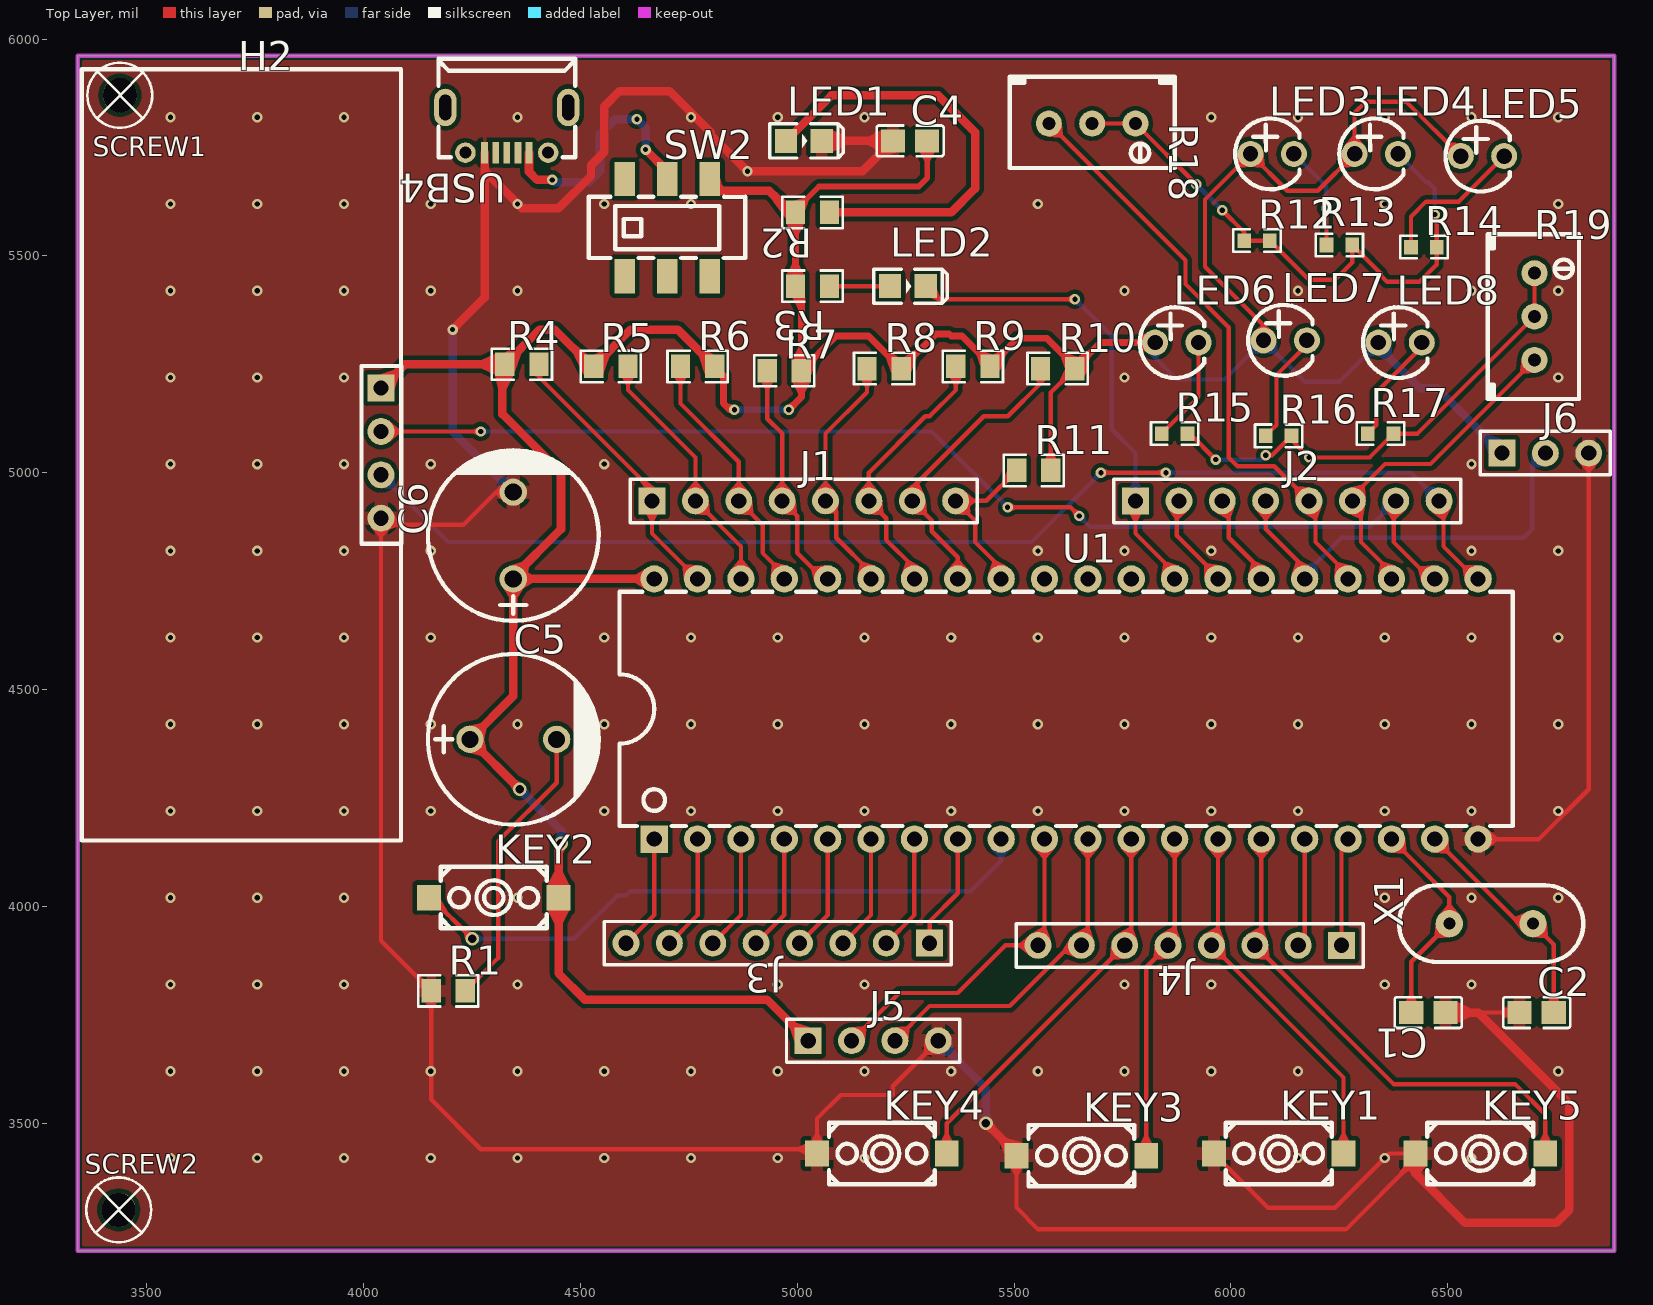
[diagram p0: Top Layer view]
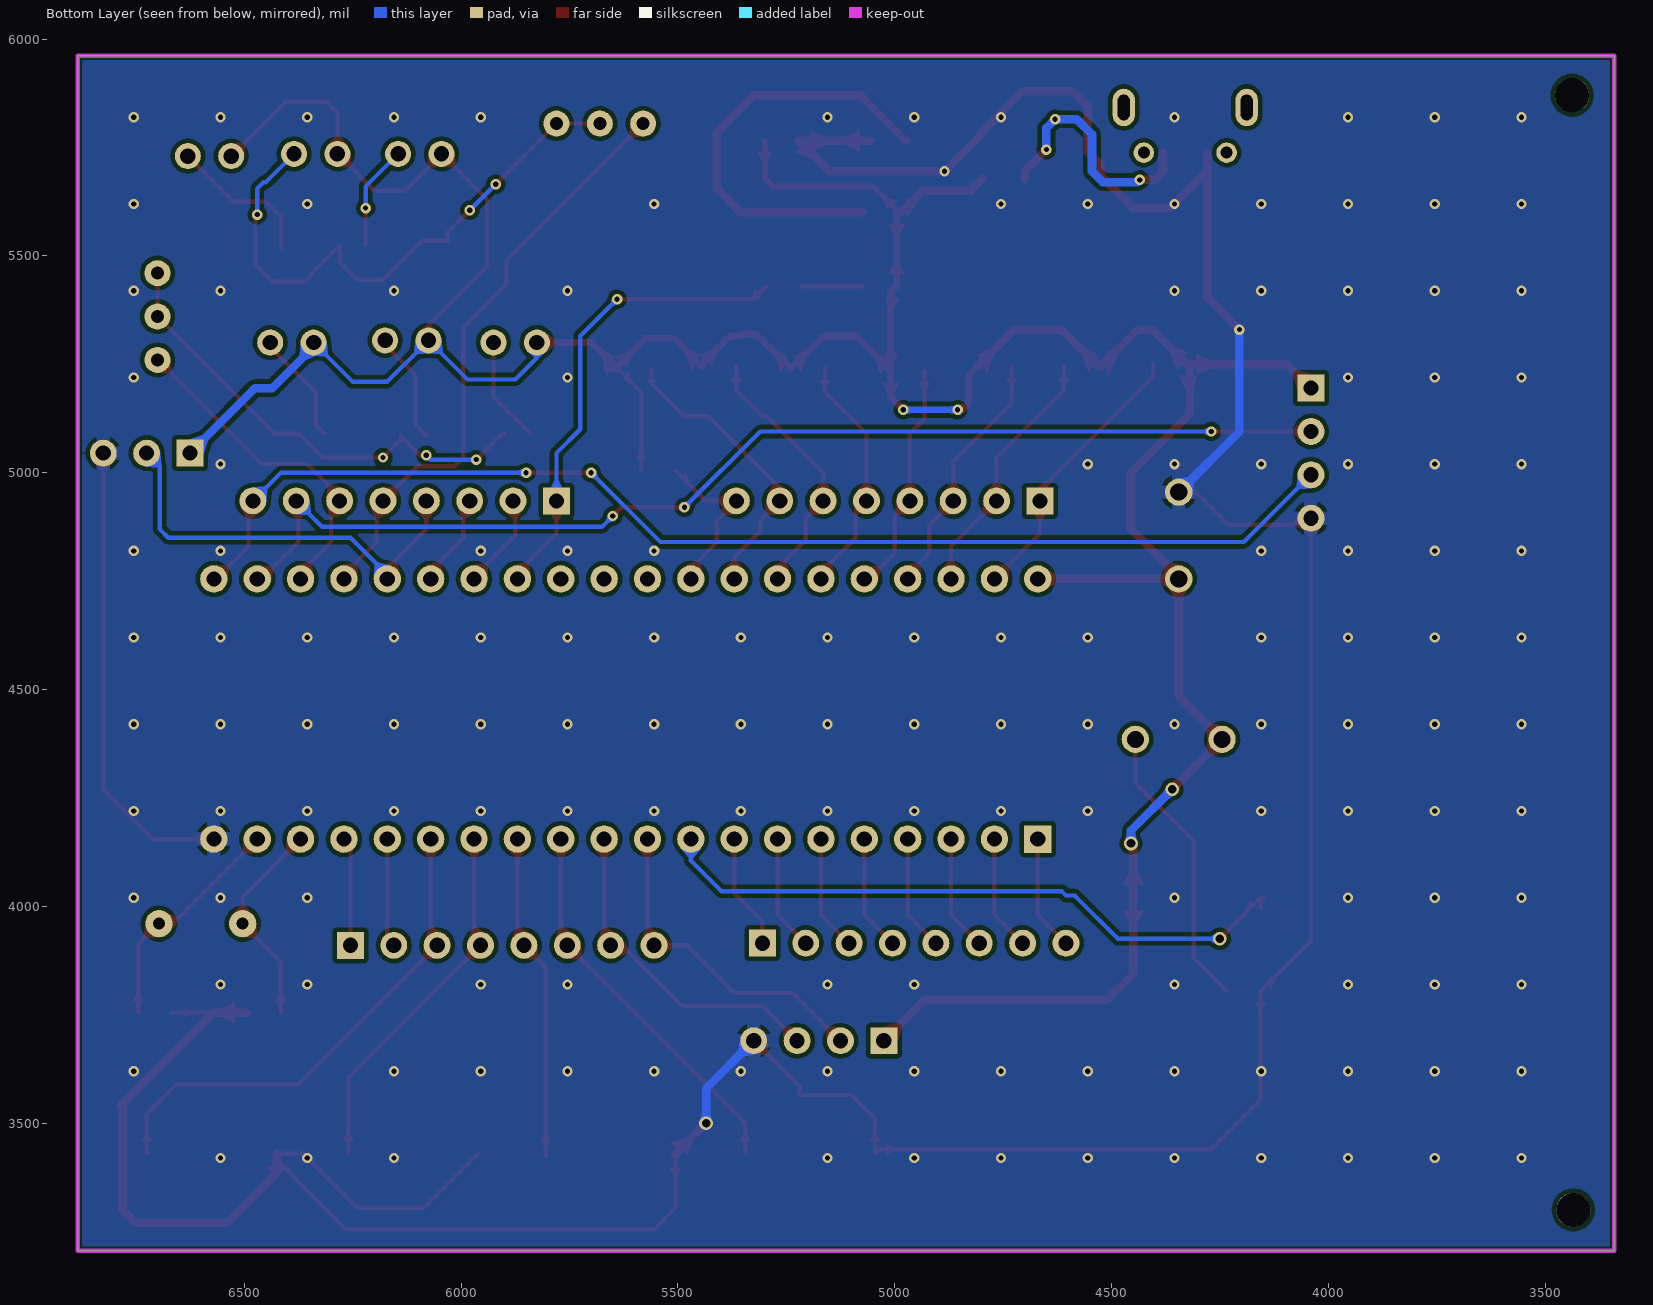
[diagram p1: Bottom Layer view, seen from below]
# Altium PCB MISC49914.pcbdoc
Units mil, origin at the board's own origin, x right, y up, seen from the top; angles counter-clockwise.
Board outline 3543.3 x 2755.9 mil, 2 copper layers (Top Layer, Bottom Layer), stack 62.206 mil thick; 50 components, 48 nets, 178 pads, 169 vias.

## Layer stack, top to bottom
Top Solder Mask Layer: solder mask 0.394, Dk 3.3
Top Layer: signal copper 1.379
Dielectric1: surface 59.449, FR4, Dk 4.5
Bottom Layer: signal copper 1.378
Bottom Solder Mask Layer: solder mask 0.394, Dk 3.3

## Board outline
3340.59,3205.55 3340.59,5961.45 6883.89,5961.45 6883.89,3205.55

## Design rules (kind name [scope] priority, off if disabled: settings)
BoardOutlineClearance Power_1 [All] p2 off: genericclearance=11.81 ignorepadtopadclearanceinfootprint=FALSE except(0: Text-CutoutEdge Arc-SplitContinuation Track-SplitContinuation SMDPad-SplitContinuation THPad-SplitContinuation Via-SplitContinuation Fill-SplitContinuation Region-SplitContinuation Poly-SplitContinuation Text-SplitContinuation Hole-SplitContinuation; 5.98: Arc-OutlineEdge Track-OutlineEdge SMDPad-OutlineEdge THPad-OutlineEdge Via-OutlineEdge Fill-OutlineEdge Region-OutlineEdge Text-OutlineEdge Hole-OutlineEdge; 10: Poly-OutlineEdge Poly-CutoutEdge; 11.81: Arc-CutoutEdge Track-CutoutEdge SMDPad-CutoutEdge THPad-CutoutEdge Via-CutoutEdge Fill-CutoutEdge Region-CutoutEdge Hole-CutoutEdge)
BoardOutlineClearance Plane_Default_1 [All] p4 off: genericclearance=5.98 ignorepadtopadclearanceinfootprint=FALSE except(0: Text-CutoutEdge Arc-SplitContinuation Track-SplitContinuation SMDPad-SplitContinuation THPad-SplitContinuation Via-SplitContinuation Fill-SplitContinuation Region-SplitContinuation Poly-SplitContinuation Text-SplitContinuation Hole-SplitContinuation; 5.98: Arc-OutlineEdge Track-OutlineEdge SMDPad-OutlineEdge THPad-OutlineEdge Via-OutlineEdge Fill-OutlineEdge Region-OutlineEdge Poly-OutlineEdge Text-OutlineEdge Hole-OutlineEdge Arc-CutoutEdge Track-CutoutEdge SMDPad-CutoutEdge THPad-CutoutEdge Via-CutoutEdge Fill-CutoutEdge Region-CutoutEdge Poly-CutoutEdge Hole-CutoutEdge)
BoardOutlineClearance Plane_Power_1 [All] p6 off: genericclearance=5.98 ignorepadtopadclearanceinfootprint=FALSE except(0: Text-CutoutEdge Arc-SplitContinuation Track-SplitContinuation SMDPad-SplitContinuation THPad-SplitContinuation Via-SplitContinuation Fill-SplitContinuation Region-SplitContinuation Poly-SplitContinuation Text-SplitContinuation Hole-SplitContinuation; 5.98: Arc-OutlineEdge Track-OutlineEdge SMDPad-OutlineEdge THPad-OutlineEdge Via-OutlineEdge Fill-OutlineEdge Region-OutlineEdge Poly-OutlineEdge Text-OutlineEdge Hole-OutlineEdge Arc-CutoutEdge Track-CutoutEdge SMDPad-CutoutEdge THPad-CutoutEdge Via-CutoutEdge Fill-CutoutEdge Region-CutoutEdge Poly-CutoutEdge Hole-CutoutEdge)
BoardOutlineClearance Copper_gge8343_1 [All] p8 off: genericclearance=5.98 ignorepadtopadclearanceinfootprint=FALSE except(0: Text-CutoutEdge Arc-SplitContinuation Track-SplitContinuation SMDPad-SplitContinuation THPad-SplitContinuation Via-SplitContinuation Fill-SplitContinuation Region-SplitContinuation Poly-SplitContinuation Text-SplitContinuation Hole-SplitContinuation; 5.98: Arc-OutlineEdge Track-OutlineEdge SMDPad-OutlineEdge THPad-OutlineEdge Via-OutlineEdge Fill-OutlineEdge Region-OutlineEdge Text-OutlineEdge Hole-OutlineEdge Arc-CutoutEdge Track-CutoutEdge SMDPad-CutoutEdge THPad-CutoutEdge Via-CutoutEdge Fill-CutoutEdge Region-CutoutEdge Hole-CutoutEdge; 10: Poly-OutlineEdge Poly-CutoutEdge)
BoardOutlineClearance Copper_gge8337_1 [All] p10 off: genericclearance=5.98 ignorepadtopadclearanceinfootprint=FALSE except(0: Text-CutoutEdge Arc-SplitContinuation Track-SplitContinuation SMDPad-SplitContinuation THPad-SplitContinuation Via-SplitContinuation Fill-SplitContinuation Region-SplitContinuation Poly-SplitContinuation Text-SplitContinuation Hole-SplitContinuation; 5.98: Arc-OutlineEdge Track-OutlineEdge SMDPad-OutlineEdge THPad-OutlineEdge Via-OutlineEdge Fill-OutlineEdge Region-OutlineEdge Text-OutlineEdge Hole-OutlineEdge Arc-CutoutEdge Track-CutoutEdge SMDPad-CutoutEdge THPad-CutoutEdge Via-CutoutEdge Fill-CutoutEdge Region-CutoutEdge Hole-CutoutEdge; 10: Poly-OutlineEdge Poly-CutoutEdge)
BoardOutlineClearance Default_1 [All] p12: genericclearance=5.98 ignorepadtopadclearanceinfootprint=FALSE except(0: Text-CutoutEdge Arc-SplitContinuation Track-SplitContinuation SMDPad-SplitContinuation THPad-SplitContinuation Via-SplitContinuation Fill-SplitContinuation Region-SplitContinuation Poly-SplitContinuation Text-SplitContinuation Hole-SplitContinuation; 5.98: Arc-OutlineEdge Track-OutlineEdge SMDPad-OutlineEdge THPad-OutlineEdge Via-OutlineEdge Fill-OutlineEdge Region-OutlineEdge Text-OutlineEdge Hole-OutlineEdge Arc-CutoutEdge Track-CutoutEdge SMDPad-CutoutEdge THPad-CutoutEdge Via-CutoutEdge Fill-CutoutEdge Region-CutoutEdge Hole-CutoutEdge; 10: Poly-OutlineEdge Poly-CutoutEdge)
Clearance Power [All] p1 off: gap=11.81 ignorepadtopadclearanceinfootprint=FALSE except(0: Text-Text; 10: Poly-Track Poly-SMDPad Poly-THPad Poly-Via Poly-Fill Poly-Region Poly-Poly Poly-Arc Poly-Text Poly-Hole)
Clearance Plane_Default [All] p3 off: gap=5.98 ignorepadtopadclearanceinfootprint=FALSE except(0: Text-Text)
Clearance Plane_Power [All] p5 off: gap=5.98 ignorepadtopadclearanceinfootprint=FALSE except(0: Text-Text; 11.81: Poly-Track Poly-SMDPad Poly-THPad Poly-Via Poly-Fill Poly-Region Poly-Poly Poly-Arc Poly-Text Poly-Hole)
Clearance Copper_gge8343 [All] p7 off: gap=5.98 ignorepadtopadclearanceinfootprint=FALSE except(0: Text-Text; 10: Poly-Track Poly-SMDPad Poly-THPad Poly-Via Poly-Fill Poly-Region Poly-Poly Poly-Arc Poly-Text Poly-Hole)
Clearance Copper_gge8337 [All] p9 off: gap=5.98 ignorepadtopadclearanceinfootprint=FALSE except(0: Text-Text; 10: Poly-Track Poly-SMDPad Poly-THPad Poly-Via Poly-Fill Poly-Region Poly-Poly Poly-Arc Poly-Text Poly-Hole)
Clearance Default [All] p11: gap=5.98 ignorepadtopadclearanceinfootprint=FALSE except(0: Text-Text; 10: Poly-Track Poly-SMDPad Poly-THPad Poly-Via Poly-Fill Poly-Region Poly-Poly Poly-Arc Poly-Text Poly-Hole)
DiffPairsRouting differentialPair [All] p1: maxlimit=6 minlimit=6 mostfreqgap=6 toplayer_minwidth=5 toplayer_prefwidth=10 toplayer_maxwidth=100 toplayer_mingap=6 toplayer_prefgap=6 toplayer_maxgap=6 bottomlayer_minwidth=5 bottomlayer_prefwidth=10 bottomlayer_maxwidth=100 bottomlayer_mingap=6 bottomlayer_prefgap=6 bottomlayer_maxgap=6 maxuncoupledlength=10
HoleToHoleClearance otherClearance [All] p1: gap=11.8 allowstackedmicrovias=TRUE
Length netLength [All] p1: minlimit=0 maxlimit=0
PasteMaskExpansion pasteMaskExpansion [All] p1: expansion=0
PlaneConnect Power_4 [All] p1 off: planeconnectstyle=Relief reliefexpansion=20 reliefentries=4 reliefconductorwidth=0 reliefairgap=10
PlaneConnect Default_4 [All] p2: planeconnectstyle=Relief reliefexpansion=20 reliefentries=4 reliefconductorwidth=0 reliefairgap=10
PolygonConnect gge8337 [All] p1 off: connectstyle=Relief reliefconductorwidth=0 reliefentries=4 polygonreliefangle="90 Angle" airgapwidth=10 via.connectstyle=Relief via.reliefconductorwidth=10 via.reliefentries=4 via.polygonreliefangle="90 Angle" via.airgapwidth=10
PolygonConnect gge8343 [All] p2: connectstyle=Relief reliefconductorwidth=0 reliefentries=4 polygonreliefangle="90 Angle" airgapwidth=10 via.connectstyle=Relief via.reliefconductorwidth=10 via.reliefentries=4 via.polygonreliefangle="90 Angle" via.airgapwidth=10
RoutingVias Power_3 [All] p1 off: holewidth=11.81 width=23.62 viastyle="Through Hole" minholewidth=11.81 minwidth=23.62 maxholewidth=2362 maxwidth=3938
RoutingVias Default_3 [All] p2: holewidth=12.01 width=23.62 viastyle="Through Hole" minholewidth=12.01 minwidth=23.62 maxholewidth=2362 maxwidth=3938
SolderMaskExpansion solderMaskExpansion [IsVia] p1: expansion=-1000 istentingtop=TRUE
SolderMaskExpansion solderMaskExpansion [All] p2: expansion=2 istentingtop=FALSE
Width Power_2 [All] p1 off: maxlimit=1000 minlimit=19.7 preferedwidth=19.7
Width Default_2 [All] p2: maxlimit=1000 minlimit=10 preferedwidth=10

## Components (designator, comment, footprint, x,y, rotation, side; value= is the part's Value field where it differs from the comment)
C1 "33p" C0805 6455,3755 r180 top
C2 "33p" C0805 6705,3755 r0 top
C4 "10NF" C0805 5260,5765 r0 top
C5 "10uF" CAP-TH_BD10.0-P5.00-D1.0-FD 4345,4385 r0 top
C6 "10uF" CAP-TH_BD10.0-P5.00-D1.0-FD 4345,4855 r90 top
H2 "HC-SR04" HC-SR04 4040,5045 r0 top
J1 "HDR-M-2.54_1x8" HDR-M-2.54_1X8 5065,4935 r0 top
J2 "HDR-M-2.54_1x8" HDR-M-2.54_1X8 6180,4935 r0 top
J3 "HDR-M-2.54_1x8" HDR-M-2.54_1X8 4905,3915 r180 top
J4 "HDR-M-2.54_1x8" HDR-M-2.54_1X8 5855,3910 r180 top
J5 "HDR-M-2.54_1x4" HDR-M-2.54_1X4 5175,3690 r0 top
J6 "HDR-M-2.54_1x3" HDR-M-2.54_1X3 6725,5045 r0 top
KEY1 "K2-3.6×6.1_SMD" KEY-SMD_2P-L6.2-W3.6-LS8.0 6110,3430 r0 top
KEY2 "K2-3.6×6.1_SMD" KEY-SMD_2P-L6.2-W3.6-LS8.0 4300,4020 r0 top
KEY3 "K2-3.6×6.1_SMD" KEY-SMD_2P-L6.2-W3.6-LS8.0 5655,3425 r0 top
KEY4 "K2-3.6×6.1_SMD" KEY-SMD_2P-L6.2-W3.6-LS8.0 5195,3430 r0 top
KEY5 "K2-3.6×6.1_SMD" KEY-SMD_2P-L6.2-W3.6-LS8.0 6575,3430 r0 top
LED1 "LED-0805_R" LED0805_RED 5015,5765 r0 top
LED2 "LED-0805_R" LED0805_RED 5255,5430 r0 top
LED3 "204-10SDRD/S530-A3-L" LED-TH_BD3.8-P2.54-FD 6095,5735 r0 top
LED4 "204-10SDRD/S530-A3-L" LED-TH_BD3.8-P2.54-FD 6335,5735 r0 top
LED5 "204-10SDRD/S530-A3-L" LED-TH_BD3.8-P2.54-FD 6580,5730 r0 top
LED6 "204-10SDRD/S530-A3-L" LED-TH_BD3.8-P2.54-FD 5875,5300 r0 top
LED7 "204-10SDRD/S530-A3-L" LED-TH_BD3.8-P2.54-FD 6125,5305 r0 top
LED8 "204-10SDRD/S530-A3-L" LED-TH_BD3.8-P2.54-FD 6390,5300 r0 top
R1 "10k" R0805 4195,3805 r0 top
R2 "1.5k" R0805 5035,5600 r180 top
R3 "1k" R0805 5035,5430 r180 top
R4 "4.7k" R0805 4365,5250 r180 top
R5 "4.7k" R0805 4570,5245 r180 top
R6 "4.7k" R0805 4770,5245 r0 top
R7 "4.7k" R0805 4970,5235 r0 top
R8 "4.7k" R0805 5200,5240 r0 top
R9 "4.7k" R0805 5405,5245 r0 top
R10 "4.7k" R0805 5600,5240 r0 top
R11 "4.7k" R0805 5545,5005 r0 top
R12 "1000" R0603 6060,5535 r0 top
R13 "1000" R0603 6250,5525 r0 top
R14 "1000" R0603 6445,5520 r0 top
R15 "1000" R0603 5870,5090 r0 top
R16 "1000" R0603 6110,5085 r0 top
R17 "1000" R0603 6345,5090 r0 top
R18 "10kΩ" RES-ADJ-TH_3296W 5680,5805 r270 top
R19 "10kΩ" RES-ADJ-TH_3296W 6700,5360 r0 top
SCREW1 "" M2螺丝 3437.7,5870.25 r0 top
SCREW2 "" M2螺丝 3435,3300 r0 top
SW2 "MST22D18G2 125" SW-SMD_MST22D18G2 4700,5565 r0 top
U1 "STC90C52RC-40I_C14023" DIP-40_L52.0-W13.7-P2.54-LS15.2-BL 5620,4455 r0 top
USB4 "USB-Micro_1" MICRO-USB-SMD_5P-P0.65-H-F_C10418 4330,5790 r180 top
X1 "11.0592MHz" OSC-TH_L10.0-W4.5-P5.00 6600,3960 r90 top

## Footprints (in the part's own frame and the unit in brackets; to place one, negate y for a bottom-side part, rotate by r counter-clockwise, add the part's x,y. Pads: shape width x height; smd on the part's side, far side on the other; paste and mask are expansions set on the pad)
C0805 [mm]
  rect 1.41x1.35 smd paste-100 mask+0.051: 1(-1,0) 2(1,0)
  silkscreen extent -1.96,-0.9 1.96,0.9
CAP-TH_BD10.0-P5.00-D1.0-FD [mm]
  round 1.6 hole 1 paste+0 mask+0.051: 1(-2.54,0) 2(2.54,0)
  silkscreen extent -5,-5 5.08,5
DIP-40_L52.0-W13.7-P2.54-LS15.2-BL [mil]
  rect 63x63 hole 35 paste+0 mask+2: 1(-950,-300)
  round 63 hole 35 paste+0 mask+2: 2(-850,-300) 3(-750,-300) 4(-650,-300) 5(-550,-300) 6(-450,-300) 7(-350,-300) 8(-250,-300) 9(-150,-300) 10(-50,-300) 11(50,-300) 12(150,-300) 13(250,-300) 14(350,-300) 15(450,-300) 16(550,-300) 17(650,-300) 18(750,-300) 19(850,-300) 20(950,-300) 21(950,300) 22(850,300) 23(750,300) 24(650,300) 25(550,300) 26(450,300) 27(350,300) 28(250,300) 29(150,300) 30(50,300) 31(-50,300) 32(-150,300) 33(-250,300) 34(-350,300) 35(-450,300) 36(-550,300) 37(-650,300) 38(-750,300) 39(-850,300) 40(-950,300)
  silkscreen extent -1030,-270 1030,270
HC-SR04 [mil]
  rect 62x62 hole 35 paste+0 mask+2: 1(0,150)
  round 62 hole 35 paste+0 mask+2: 2(0,50) 3(0,-50) 4(0,-150)
  silkscreen extent -690,-893 47,885
HDR-M-2.54_1X3 [mil]
  rect 62x62 hole 35 paste+0 mask+2: 1(-100,0)
  round 62 hole 35 paste+0 mask+2: 2(0,0) 3(100,0)
  silkscreen extent -150,-50 150,50
HDR-M-2.54_1X4 [mil]
  rect 62x62 hole 35 paste+0 mask+2: 1(-150,0)
  round 62 hole 35 paste+0 mask+2: 2(-50,0) 3(50,0) 4(150,0)
  silkscreen extent -200,-50 200,50
HDR-M-2.54_1X8 [mil]
  rect 62x62 hole 35 paste+0 mask+2: 1(-400,0)
  round 62 hole 35 paste+0 mask+2: 2(-300,0) 3(-200,0) 4(-100,0) 5(0,0) 6(100,0) 7(200,0) 8(300,0)
  silkscreen extent -450,-50 350,50
KEY-SMD_2P-L6.2-W3.6-LS8.0 [mm]
  rect 1.4x1.5 smd paste+0 mask+0.051: 1(-3.8,0) 2(3.8,0)
  silkscreen extent -3.1,-1.8 3.1,1.8
LED0805_RED [mil]
  rect 51.2x55.1 smd paste+0 mask+2: 1(-41.35,0) 2(41.35,0)
  silkscreen extent -79,-39 91,39
LED-TH_BD3.8-P2.54-FD [mil]
  round 60 hole 35.43 paste+0 mask+2: 1(-50,0) 2(50,0)
  silkscreen extent -85,-82 63,82
M2螺丝 [mm]
  round 2 hole 2: 1(0,0)
  silkscreen extent -1.9,-1.9 1.9,1.9
MICRO-USB-SMD_5P-P0.65-H-F_C10418 [mm]
  rect 0.4x1.25 smd paste-100 mask+0.051: 1(-1.3,1.325) 2(-0.65,1.325) 3(0,1.325) 4(0.65,1.325) 5(1.3,1.325)
  round 1.2 hole 0.7 paste+0 mask+0.051: SH0(-2.425,1.325) SH3(2.425,1.325)
  oval 1.3x2.2 hole 0.7 slot 1.5 at 90 deg paste+0 mask+0.051: SH1(-3.6,-1.325) SH2(3.6,-1.325)
  silkscreen extent -4,-4.17 4,1.59
OSC-TH_L10.0-W4.5-P5.00 [mm]
  round 1.6 hole 0.7 paste+0 mask+0.051: 1(0,2.45) 2(0,-2.45)
  silkscreen extent -2.25,-5.39 2.25,5.39
R0603 [mil]
  rect 31.75x34.02 smd paste-3937.01 mask+2: 1(-29.66,0) 2(29.66,0)
  silkscreen extent -55,-26 55,26
R0805 [mm]
  rect 1.133x1.377 smd paste-100 mask+0.051: 1(-1,0) 2(1,0)
  silkscreen extent -1.76,-0.92 1.76,0.92
RES-ADJ-TH_3296W [mil]
  round 60 hole 30 paste+0 mask+2: 1(0,99.99) 2(0,-0.01) 3(0,-100.01)
  silkscreen extent -108,-190 102,190
SW-SMD_MST22D18G2 [mm]
  rect 1.2x2 smd paste+0 mask+0.051: 1(-2.5,2.85) 2(0,2.85) 3(2.5,2.85) 4(-2.5,-2.85) 5(0,-2.85) 6(2.5,-2.85)
  silkscreen extent -4.6,-1.78 4.57,1.8

## Via types
v1: diameter 23.62, hole 12, Top Layer to Bottom Layer, 145 vias
v2: diameter 24, hole 12, Top Layer to Bottom Layer, 20 vias
v3: diameter 31.5, hole 19.7, Top Layer to Bottom Layer, 4 vias

## Nets (pads, with @x,y where several pads share a name; then routed paths per layer and width w, separated by ;. In a path a pad name is that pad's centre, name@x,y a point inside that pad or via, vN(x,y) a via of type N, cw(c..) or ccw(c..) an arc to the next point about the centre after c; other vN are vias at no path point)
$1N75: J3.8 U1.1 | length 266.9
  Top Layer w10: J3.8 4670,3980 U1.1
$1N76: J3.7 U1.2 | length 266.9
  Top Layer w10: J3.7 4770,3980 U1.2
$1N77: J3.6 U1.3 | length 266.9
  Top Layer w10: J3.6 4870,3980 U1.3
$1N78: J3.5 U1.4 | length 266.9
  Top Layer w10: J3.5 4970,3980 U1.4
$1N79: J3.4 U1.5 | length 266.9
  Top Layer w10: J3.4 5070,3980 U1.5
$1N80: J3.3 U1.6 | length 266.9
  Top Layer w10: J3.3 5170,3980 U1.6
$1N81: J3.2 U1.7 | length 266.9
  Top Layer w10: J3.2 5270,3980 U1.7
$1N82: J3.1 U1.8 | length 266.9
  Top Layer w10: J3.1 5305,3965 5370,4030 U1.8
$1N95: J4.2 U1.16 | length 251.2
  Top Layer w10: J4.2 6170,3925 U1.16
$1N96: J4.1 U1.17 | length 251.2
  Top Layer w10: J4.1 6255,4140 U1.17
$1N164: SW2.2 USB4.1 | length 579.3
  Top Layer w19.68: USB4.1 4381.2,5693.8 4400,5675 v2(4435,5675) ; v2(4650,5745) 4700,5695 SW2.2
  Bottom Layer w19.68: v2(4435,5675) 4440,5670 4520,5670 4545,5695 4545,5780 4580,5815 v2(4630,5815) 4650,5795 v2(4650,5745)
$1N297: LED1.1 R2.1 | length 1003.4
  Top Layer w19.68: LED1.1@4973.7,5765 5078.7,5870 5325,5870 5410,5785 5410,5655 5355,5600 R2.1
$1N368: LED2.1 R3.1 | length 139.3
  Top Layer w10: R3.1 LED2.1@5213.7,5430
$1N557: LED4.2 R12.1 R12.2 R13.2 R14.2 R18.1 R18.2 | length 1361.9
  Top Layer w10: R18.2 R18.1 v2(5920,5665) ; v2(5980,5605) 6030.3,5554.7 R12.1 R12.2 6179.7,5445 6240,5445 6279.7,5484.7 R13.2 6345,5459.7 6345,5455 6360,5440 6435,5440 6474.7,5479.7 R14.2 6474.7,5590.3 v2(6470,5595)
  Bottom Layer w10: v2(5920,5665) v2(5980,5605) ; LED4.2 6450,5670 6455,5670 6470,5655 v2(6470,5595)
$1N566: LED3.2 R13.1 | length 241.1
  Top Layer w10: v2(6220,5610) R13.1
  Bottom Layer w10: LED3.2 6220,5660 v2(6220,5610)
$1N604: LED5.2 R14.1 | length 342.9
  Top Layer w10: R14.1 6415.3,5590.3 6450,5625 6525,5625 LED5.2
$1N665: LED8.2 R17.1 | length 261.7
  Top Layer w10: R17.1 6335,5109.7 6335,5185 6440,5290 LED8.2
$1N666: LED7.2 R16.1 | length 259.2
  Top Layer w10: R16.1 6105,5109.7 6105,5225 6175,5295 LED7.2
$1N673: R15.2 R16.2 R17.2 R19.1 R19.2 | length 1108.9
  Top Layer w10: R15.2 5905,5090 v2(5965,5030) ; v2(6080,5040) 6094.7,5040 R16.2 6139.7,5075.3 v2(6180,5035) 6319.7,5035 R17.2 6430,5090 R19.2 R19.1
  Bottom Layer w10: v2(5965,5030) 6070,5030 v2(6080,5040)
$1N675: LED6.2 R15.1 | length 245.1
  Top Layer w10: R15.1 5925,5174.7 LED6.2
$1N776: C5.2 R1.2 | length 667.2
  Top Layer w10: R1.2 4310,3880.6 4310,4150 4445,4285 C5.2
+5V: C4.2 C5.1 C6.1 H2.1 J5.1 J6.1 KEY2.2 LED3.1 LED4.1 LED5.1 LED6.1 LED7.1 LED8.1 R2.2 R3.2 R4.2 R5.2 R6.2 R7.2 R8.2 R9.2 R10.2 R11.2 SW2.3 U1.40 | length 8572.5
  Top Layer w10: R11.2 5584.4,5185 R10.2 ; LED7.1 6075,5340 5940,5475 5940,5630 LED3.1 6130,5650 6200,5650 LED4.1 6285,5830 6310,5855 6405,5855 LED5.1
  Top Layer w13: R2.2 4995.6,5605.6 5050,5660 5280,5660 5300,5680 C4.2
  Top Layer w15.75: R6.2 4830,5224.4 4830,5160 4845,5145 v2(4855,5145) ; v2(4980,5145) 5009.4,5174.4 R7.2 ; R2.2 R3.2 5009.4,5416.3 R7.2 ; LED6.1 5699.4,5300 R10.2 5660,5240 5665,5245 5640,5245 5575,5310 5509.4,5310 R9.2 5444.4,5250.6 5380,5315 5355,5315 5350,5320 5319.4,5320 R8.2 5164.4,5315 5089.4,5315 R7.2
  Top Layer w19.68: H2.1 4095,5250 R4.2 ; v3(4360,4270) C5.1 4345,4485 C6.1 ; v3(4455,4145) 4449.6,4139.6 KEY2.2 4449.6,3845.4 4510,3785 4930,3785 J5.1 ; U1.40 C6.1 ; SW2.3 4825.6,5650 4935,5650 4985,5600 R2.2 ; R6.2 4724.4,5330 4615.6,5330 R5.2 4525,5245 4440,5330 4405.6,5330 R4.2 ; R4.2 4320,5244.4 4320,5135 4455,5000 4455,4870 4345,4760 C6.1
  Bottom Layer w10: LED6.1 5825,5265 5875,5215 5985,5215 LED7.1 6170,5210 6250,5210 LED8.1
  Bottom Layer w15.75: v2(4855,5145) v2(4980,5145)
  Bottom Layer w19.68: v3(4360,4270) 4455,4175 v3(4455,4145) ; LED8.1 6340,5290 6435,5195 6475,5195 J6.1
GND: C1.1 C2.1 C4.1 C6.2 H2.4 J5.4 J6.3 KEY1.1 KEY3.1 KEY4.1 KEY5.1 LED1.2 R1.1 U1.20 USB4.5 | length 9845
  Top Layer w10: C6.2 4305,4955 4230,4880 4055,4880 H2.4 4040,3920.6 R1.1 4155.6,3554.4 4270,3440 5035.4,3440 KEY4.1 5045.4,3510.4 5100,3565 5220,3565 5220,3585 J5.4 ; KEY3.1 5505.4,3305.4 5555,3255 6265,3255 6425.4,3415.4 KEY5.1 6365,3430 6354.67,3419.67 6240,3305 6085.4,3305 KEY1.1 ; C1.1 C2.1 ; U1.20@6575,4155 6710,4155 6825,4270 J6.3
  Top Layer w19.68: v2(4205,5330) 4278.8,5403.8 USB4.5 4278.8,5696.2 4365,5610 4450,5610 4525,5685 4525,5710 4555,5740 4555,5845 4590,5880 4705,5880 4800,5785 4800,5780 v2(4885,5695) 5150.6,5695 C4.1 LED1.2@5056.3,5765 ; v3(5435,3500) 5505.4,3429.6 KEY3.1 ; KEY5.1 6425.4,3384.6 6540,3270 6750,3270 6780,3300 6780,3535 6785,3540 6570,3755 C1.1
  Bottom Layer w19.68: v2(4205,5330) 4205,5095 C6.2 ; J5.4 5435,3580 v3(5435,3500)
  other v1: 3554.69,3419.65 3754.69,3419.65 3954.69,3419.65 4154.69,3419.65 4354.69,3419.65 4554.69,3419.65 4754.69,3419.65 4954.69,3419.65 5154.69,3419.65 6154.69,3419.65 6354.69,3419.65 6554.69,3419.65 3554.69,3619.65 3754.69,3619.65 3954.69,3619.65 4154.69,3619.65 4354.69,3619.65 4554.69,3619.65 4754.69,3619.65 4954.69,3619.65 5154.69,3619.65 5354.69,3619.65 5554.69,3619.65 5754.69,3619.65 5954.69,3619.65 6154.69,3619.65 6754.69,3619.65 3554.69,3819.65 3754.69,3819.65 3954.69,3819.65 4354.69,3819.65 4954.69,3819.65 5154.69,3819.65 5754.69,3819.65 5954.69,3819.65 6354.69,3819.65 6554.69,3819.65 3554.69,4019.65 3754.69,4019.65 3954.69,4019.65 4354.69,4019.65 6354.69,4019.65 6554.69,4019.65 6754.69,4019.65 3554.69,4219.65 3754.69,4219.65 3954.69,4219.65 4154.69,4219.65 4554.69,4219.65 4754.69,4219.65 4954.69,4219.65 5154.69,4219.65 5354.69,4219.65 5554.69,4219.65 5754.69,4219.65 5954.69,4219.65 6154.69,4219.65 6354.69,4219.65 6554.69,4219.65 6754.69,4219.65 3554.69,4419.65 3754.69,4419.65 3954.69,4419.65 4154.69,4419.65 4354.69,4419.65 4554.69,4419.65 4754.69,4419.65 4954.69,4419.65 5154.69,4419.65 5354.69,4419.65 5554.69,4419.65 5754.69,4419.65 5954.69,4419.65 6154.69,4419.65 6354.69,4419.65 6554.69,4419.65 6754.69,4419.65 3554.69,4619.65 3754.69,4619.65 3954.69,4619.65 4154.69,4619.65 4554.69,4619.65 4754.69,4619.65 4954.69,4619.65 5154.69,4619.65 5354.69,4619.65 5554.69,4619.65 5754.69,4619.65 5954.69,4619.65 6154.69,4619.65 6354.69,4619.65 6554.69,4619.65 6754.69,4619.65 3554.69,4819.65 3754.69,4819.65 3954.69,4819.65 4154.69,4819.65 5554.69,4819.65 5754.69,4819.65 5954.69,4819.65 6554.69,4819.65 6754.69,4819.65 3554.69,5019.65 3754.69,5019.65 3954.69,5019.65 4154.69,5019.65 4354.69,5019.65 4554.69,5019.65 6554.69,5019.65 3554.69,5219.65 3754.69,5219.65 3954.69,5219.65 5754.69,5219.65 6754.69,5219.65 3554.69,5419.65 3754.69,5419.65 3954.69,5419.65 4154.69,5419.65 4354.69,5419.65 5754.69,5419.65 6154.69,5419.65 6554.69,5419.65 6754.69,5419.65 3554.69,5619.65 3754.69,5619.65 3954.69,5619.65 4154.69,5619.65 4354.69,5619.65 4554.69,5619.65 4754.69,5619.65 5554.69,5619.65 6354.69,5619.65 6754.69,5619.65 3554.69,5819.65 3754.69,5819.65 3954.69,5819.65 4354.69,5819.65 4754.69,5819.65 4954.69,5819.65 5154.69,5819.65 5954.69,5819.65 6154.69,5819.65 6354.69,5819.65 6554.69,5819.65 6754.69,5819.65
P0.0: J1.1 R4.1 U1.39 | length 646.4
  Top Layer w10: R4.1 4404.4,5220.6 4665,4960 J1.1 4665,4860 U1.39
P0.1: J1.2 R5.1 U1.38 | length 597.9
  Top Layer w10: R5.1 4609.4,5190.6 4765,5035 J1.2 4870,4830 U1.38
P0.2: J1.3 R6.1 U1.37 | length 589.2
  Top Layer w10: R6.1 4730.6,5159.4 4865,5025 J1.3 4920,4880 4920,4815 4970,4765 U1.37
P0.3: J1.4 R7.1 U1.36 | length 543.6
  Top Layer w10: R7.1 4930.6,5124.4 4965,5090 J1.4 5000,4900 5000,4815 5060,4755 U1.36
P0.4: J1.5 R8.1 U1.35 | length 568.1
  Top Layer w10: R8.1 5160.6,5185.6 5065,5090 J1.5 5090,4910 5090,4850 5170,4770 U1.35
P0.5: J1.6 R9.1 U1.34 | length 622.4
  Top Layer w10: U1.34 5270,4780 5205,4845 5205,4895 J1.6 5165,5000 5295,5130 5305,5130 5365.6,5190.6 R9.1
P0.6: J1.7 R10.1 U1.33 | length 683.2
  Top Layer w10: U1.33 5370,4805 5310,4865 5310,4890 J1.7 5265,4965 5430,5130 5485,5130 5560.6,5205.6 R10.1
P0.7: J1.8 R11.1 U1.32 | length 393.1
  Top Layer w10: U1.32 5470,4780 5410,4840 5410,4890 J1.8 5435.6,4935 R11.1
P2.0: H2.3 J2.8 U1.21 | length 2817.6
  Top Layer w10: v2(5700,5000) v2(5850,5000) ; J2.8 6490,4925 6490,4830 6565,4755 U1.21
  Bottom Layer w10: H2.3 4195,4840 5540,4840 v2(5700,5000) ; v2(5850,5000) 6415,5000 J2.8
P2.1: H2.2 J2.7 U1.22 | length 2683.3
  Top Layer w10: H2.2 v2(4270,5095) ; v2(5485,4920) 5630,4920 v2(5650,4900) ; J2.7 6375,4930 6375,4840 6460,4755 U1.22
  Bottom Layer w10: v2(4270,5095) 5310,5095 v2(5485,4920) ; v2(5650,4900) 5675,4875 6215,4875 6320,4875 J2.7
P2.2: J2.6 R19.3 U1.23 | length 777.8
  Top Layer w10: U1.23 6370,4770 6300,4840 6300,4915 J2.6 6280,4945 6355,5020 6460,5020 R19.3
P2.3: J2.5 R18.3 U1.24 | length 1385.6
  Top Layer w10: R18.3 5895,5490 5895,5435 5995,5335 5995,5035 6015,5015 6100,5015 J2.5 6195,4920 6195,4840 6270,4765 U1.24
P2.4: J2.4 J6.2 U1.25 | length 983.2
  Top Layer w10: J2.4 6080,4870 6170,4780 U1.25
  Bottom Layer w10: U1.25 6170,4765 6255,4850 6675,4850 6695,4870 6695,5015 J6.2
P2.5: J2.3 U1.26 | length 217.3
  Top Layer w10: J2.3 5995,4920 5995,4850 6070,4775 U1.26
P2.6: J2.2 U1.27 | length 221.4
  Top Layer w10: J2.2 5875,4930 5875,4855 5970,4760 U1.27
P2.7: J2.1 LED2.2 U1.28 | length 1096.4
  Top Layer w10: LED2.2@5296.3,5430 5326.3,5400 v2(5640,5400) ; J2.1 5780,4860 5870,4770 U1.28
  Bottom Layer w10: v2(5640,5400) 5725,5315 5725,5100 5780,5045 J2.1
P3.2: J4.6 KEY4.2 U1.12 | length 901.2
  Top Layer w10: KEY4.2 5344.6,3499.6 J4.6 5770,3925 U1.12
P3.3: J4.5 KEY3.2 U1.13 | length 757.1
  Top Layer w10: KEY3.2 5804.6,3859.6 J4.5 5870,3925 U1.13
P3.4: J4.4 KEY1.2 U1.14 | length 857.4
  Top Layer w10: U1.14 5970,3925 J4.4 6259.6,3605.4 KEY1.2
P3.5: J4.3 KEY5.2 U1.15 | length 1172.6
  Top Layer w10: U1.15 6070,3925 J4.3 6375,3590 6655,3590 6724.6,3520.4 KEY5.2
RST: KEY2.1 U1.9 | length 1515.8
  Top Layer w10: KEY2.1@4155.62,3994.84 4155.62,4014.77 KEY2.1 4155.4,4020 v3(4250.37,3925)
  Bottom Layer w10: v3@4245.4,3925 4485,3925 4585,4025 4605,4025 4615,4035 5400,4035 5470,4105 U1.9
RXD: J4.8 J5.2 U1.10 | length 772.3
  Top Layer w10: J5.2 5235,3800 5370,3800 5480,3910 J4.8 5570,3925 U1.10
TXD: J4.7 J5.3 U1.11 | length 772.3
  Top Layer w10: J5.3 5305,3770 5490,3770 5630,3910 J4.7 5670,3925 U1.11
XTAL1: C2.2 U1.19 X1.2 | length 532.1
  Top Layer w10: U1.19 6665,3960 X1.2 ; X1.2 6744.4,3912.1 C2.2
XTAL2: C1.2 U1.18 X1.1 | length 491.7
  Top Layer w10: U1.18 6503.54,4021.46 X1.1 ; C1.2 6415.6,3872.1 X1.1
pads on no net: SCREW1.1 SCREW2.1 SW2.1 SW2.4 SW2.5 SW2.6 U1.29 U1.30 U1.31 USB4.2 USB4.3 USB4.4 USB4.SH0 USB4.SH1 USB4.SH2 USB4.SH3

## Polygon pours and split planes (outlines as drawn)
GND on Bottom Layer (solid, remove dead copper, pour order 4): 3240,6120 3245,6115 6985,6115 7075,6025 7075,3075 7000,3000 3110,3000 3015,3095 3015,3260 3015,3270
GND on Top Layer (solid, remove dead copper, pour order 0): 3000,6085 3040,6045 6965,6045 6995,6015 6995,3115 6990,3120 3125,3120 3105,3140 3105,3200

## Keep-outs
Board Outline Layer:
  the board outline again, w10

## Other copper
Top Layer:
  region net +5V: 4243.03,4353.57 4268.36,4347.72 4282.28,4361.64 4276.43,4386.97
  region net +5V: 4243.03,4416.43 4276.43,4383.03 4282.28,4408.36 4268.36,4422.28
  region net +5V: 4368.62,4734.17 4321.38,4734.17 4335.16,4712.12 4354.84,4712.12
  region net +5V: 4365.83,4731.38 4387.88,4745.16 4387.88,4764.84 4365.83,4778.62
  region net +5V: 4376.49,4755.63 4380.25,4781.33 4365.18,4794.1 4340.44,4786.16
  region net GND: 4324.17,4931.38 4324.17,4978.62 4305,4960 4305,4950
  region net GND: 4067.43,4909.44 4050.9,4865.98 4077.55,4875 4081.35,4885
  region net GND: 4063.25,4874.5 4016.75,4874.5 4035,4852.8 4045,4852.8
  region net P2.1: 4060.5,5071.75 4082.2,5090 4082.2,5100 4060.5,5118.25
  region net P0.1: 4763.06,4904.06 4791.31,4901.62 4798.38,4908.69 4795.94,4936.94
  region net P0.1: 4788.25,4955.5 4770,4977.2 4760,4977.2 4741.75,4955.5
  region net P0.2: 4863.06,4904.06 4891.31,4901.62 4898.38,4908.69 4895.94,4936.94
  region net P0.2: 4888.25,4955.5 4870,4977.2 4860,4977.2 4841.75,4955.5
  region net P0.3: 4963.06,4904.06 4991.31,4901.62 4998.38,4908.69 4995.94,4936.94
  region net P0.3: 4988.25,4955.5 4970,4977.2 4960,4977.2 4941.75,4955.5
  region net P0.4: 5063.06,4904.06 5086.46,4906.46 5093.54,4913.54 5095.94,4936.94
  region net P0.4: 5088.25,4955.5 5070,4977.2 5060,4977.2 5041.75,4955.5
  region net P0.5: 5163.06,4904.06 5191.31,4901.62 5198.38,4908.69 5195.94,4936.94
  region net P0.5: 5188.25,4955.5 5170,4977.2 5160,4977.2 5141.75,4955.5
  region net P0.6: 5263.06,4904.06 5291.31,4901.62 5298.38,4908.69 5295.94,4936.94
  region net P0.6: 5292.72,4948.87 5281.39,4974.32 5270.21,4977.28 5247.77,4960.77
  region net P0.7: 5385.5,4911.75 5407.2,4930 5407.2,4940 5385.5,4958.25
  region net P0.7: 5363.06,4904.06 5391.31,4901.62 5398.38,4908.69 5395.94,4936.94
  region net P2.6: 5900.66,4911.89 5854.48,4917.39 5870,4893.69 5880,4892.5
  region net P2.5: 6009.02,4924.1 5965.56,4907.57 5990,4893.65 6000,4897.45
  region net P2.4: 6103.25,4914.5 6056.75,4914.5 6075,4892.8 6085,4892.8
  region net P2.3: 6209.02,4924.1 6165.56,4907.57 6190,4893.65 6200,4897.45
  region net P2.3: 6149.06,4933.06 6181.94,4965.94 6153.69,4968.38 6146.62,4961.31
  region net P2.2: 6310.19,4927.96 6269.24,4905.93 6295,4895.14 6305,4900.53
  region net P2.2: 6310.83,4938.27 6308.56,4966.49 6300.28,4972.36 6272.9,4965.18
  region net P2.1: 6400.66,4911.89 6354.48,4917.39 6370,4893.69 6380,4892.5
  region net P2.0: 6462.27,4909.57 6485,4892.78 6495,4895.22 6507.45,4920.59
  region net P3.5: 6084.02,3920.9 6075,3947.55 6065,3951.35 6040.56,3937.43
  region net P3.5: 6053.06,3879.06 6081.31,3876.62 6088.38,3883.69 6085.94,3911.94
  region net P3.4: 5984.02,3920.9 5975,3947.55 5965,3951.35 5940.56,3937.43
  region net P3.4: 5953.06,3879.06 5981.31,3876.62 5988.38,3883.69 5985.94,3911.94
  region net P3.3: 5884.02,3920.9 5875,3947.55 5865,3951.35 5840.56,3937.43
  region net P3.3: 5824.06,3911.94 5821.62,3883.69 5828.69,3876.62 5856.94,3879.06
  region net P3.2: 5784.02,3920.9 5775,3947.55 5765,3951.35 5740.56,3937.43
  region net P3.2: 5724.06,3911.94 5721.62,3883.69 5728.69,3876.62 5756.94,3879.06
  region net TXD: 5643.8,3881.09 5627.72,3924.72 5613.5,3900.57 5617.31,3890.23
  region net TXD: 5684.02,3920.9 5675,3947.55 5665,3951.35 5640.56,3937.43
  region net RXD: 5584.02,3920.9 5575,3947.55 5565,3951.35 5540.56,3937.43
  region net RXD: 5534.5,3886.75 5534.5,3933.25 5512.8,3915 5512.8,3905
  region net RXD: 5123.06,3720.94 5155.94,3688.06 5158.38,3716.31 5151.31,3723.38
  region net TXD: 5223.06,3720.94 5255.94,3688.06 5258.38,3716.31 5251.31,3723.38
  region net GND: 5294.06,3691.94 5291.62,3663.69 5298.69,3656.62 5326.94,3659.06
  region net GND: 6848.25,5024.5 6801.75,5024.5 6820,5002.8 6830,5002.8
  region net +5V: 6043.12,5705.06 6070.34,5702.58 6077.42,5709.66 6074.94,5736.88
  region net +5V: 6015.06,5736.88 6012.58,5709.66 6019.66,5702.58 6046.88,5705.06
  region net +5V: 6307.5,5754.84 6290,5775.84 6280,5775.84 6262.5,5754.84
  region net +5V: 6255.06,5736.88 6252.58,5709.66 6259.66,5702.58 6286.88,5705.06
  region net +5V: 6500.06,5728.12 6531.88,5759.94 6504.66,5762.42 6497.58,5755.34
  region net +5V: 5805.16,5277.5 5805.16,5322.5 5784.16,5307.87 5784.16,5292.13
  region net +5V: 6097.5,5324.84 6080,5340 6070,5340 6052.5,5324.84
  region net P2.3: 5578.12,5775.06 5605.34,5772.58 5612.41,5779.65 5609.94,5806.88
  region net P2.2: 6670.06,5261.88 6667.58,5234.66 6674.66,5227.58 6701.88,5230.06
  region net P0.7: 5484.76,4782.83 5460.01,4797.06 5449.74,4793.19 5440.54,4766.16
  region net P0.6: 5393.62,4775.84 5375,4797.89 5365,4797.89 5346.38,4775.84
  region net P2.7: 5879.69,4784.97 5852.56,4794.52 5843.68,4789.25 5839.05,4760.86
  region net P0.5: 5284.76,4782.83 5260.01,4797.06 5249.74,4793.19 5240.54,4766.16
  region net P2.6: 5974.56,4786.17 5946.11,4790.96 5938.45,4784.48 5938.51,4755.63
  region net P0.4: 5179.69,4784.97 5152.56,4794.52 5143.68,4789.25 5139.05,4760.86
  region net P2.5: 6082.23,4784.03 6056.14,4795.93 6046.6,4791.33 6039.67,4763.51
  region net P2.4: 6184.76,4782.83 6160.01,4797.06 6149.74,4793.19 6140.54,4766.16
  region net P2.3: 6277.13,4785.68 6249.22,4792.85 6240.96,4786.96 6238.67,4758.24
  region net P0.3: 5066.76,4786.33 5038.04,4784.04 5032.15,4775.78 5039.32,4747.87
  region net P0.2: 4977.13,4785.68 4949.22,4792.85 4940.96,4786.96 4938.67,4758.24
  region net P2.2: 6379.69,4784.97 6352.56,4794.52 6343.68,4789.25 6339.05,4760.86
  region net P2.1: 6466.76,4786.33 6438.04,4784.04 6432.15,4775.78 6439.32,4747.87
  region net P2.0: 6569.37,4786.49 6540.52,4786.55 6534.04,4778.89 6538.83,4750.44
  region net P0.1: 4893.62,4775.84 4875,4797.89 4865,4797.89 4846.38,4775.84
  region net P0.0: 4738.56,4753.03 4771.97,4786.44 4743.21,4788.86 4736.14,4781.79
  region net +5V: 4649.16,4731.38 4649.16,4778.62 4627.11,4764.84 4627.11,4745.16
  region net RXD: 5593.62,4134.16 5546.38,4134.16 5565,4112.11 5575,4112.11
  region net TXD: 5693.62,4134.16 5646.38,4134.16 5665,4112.11 5675,4112.11
  region net P3.2: 5793.62,4134.16 5746.38,4134.16 5765,4112.11 5775,4112.11
  region net P3.3: 5893.62,4134.16 5846.38,4134.16 5865,4112.11 5875,4112.11
  region net P3.4: 5993.62,4134.16 5946.38,4134.16 5965,4112.11 5975,4112.11
  region net P3.5: 6093.62,4134.16 6046.38,4134.16 6065,4112.11 6075,4112.11
  region net XTAL2: 6368.03,4123.56 6396.79,4121.14 6403.86,4128.21 6401.44,4156.97
  region net XTAL1: 6468.03,4123.56 6496.79,4121.14 6503.86,4128.21 6501.44,4156.97
  region net GND: 6590.84,4131.38 6612.89,4150 6612.89,4160 6590.84,4178.62
  region net XTAL1: 6681.84,3987.9 6656.2,3975.87 6653.42,3964.51 6670.61,3942.01
  region net XTAL1: 6694.49,3928.57 6723.25,3926.14 6730.32,3933.21 6727.89,3961.97
  region net XTAL2: 6527.16,3980.83 6508.54,4002.88 6498.54,4002.88 6479.92,3980.83
  region net XTAL2: 6472.11,3961.97 6469.68,3933.21 6476.75,3926.14 6505.51,3928.57
  region net GND: 4216.98,5329.25 4223.51,5334.59 4209.59,5348.51 4204.25,5341.98
  region net GND: 4885.75,5706.98 4880.41,5713.51 4866.49,5699.59 4873.02,5694.25
  region net GND: 4892.94,5686 4901.34,5685.16 4901.34,5704.84 4892.94,5704
  region net P2.7: 5632.06,5391 5632.06,5409 5623.66,5405 5623.66,5395
  region net +5V: 4850.49,5156.12 4842.48,5158.65 4836.69,5142.17 4844.53,5139.14
  region net +5V: 4991.98,5144.25 4997.12,5150.98 4985.98,5162.12 4979.25,5156.98
  region net P2.0: 5842.06,4991 5842.06,5009 5833.66,5005 5833.66,4995
  region net P2.0: 5707.94,4991 5716.34,4995 5716.34,5005 5707.94,5009
  region net P2.1: 5650.75,4911.98 5641.98,4915.09 5634.91,4908.02 5638.02,4899.25
  region net P2.1: 5492.94,4911 5501.34,4915 5501.34,4925 5492.94,4929
  region net P2.1: 4262.06,5086 4262.06,5104 4253.66,5100 4253.66,5090
  region net RST: 4251.35,3940.72 4238.74,3943.7 4231.67,3936.62 4234.65,3924.01
  region net +5V: 4360.99,4285.72 4351.8,4292.12 4337.88,4278.2 4344.28,4269.01
  region net +5V: 4463.81,4131.94 4440.95,4137.89 4439.76,4126.81 4459.44,4121.69
  region net GND: 5450.72,3500.99 5434.01,3484.28 5443.2,3477.88 5457.12,3491.8
  region net XTAL2: 6403.13,3781.57 6428.13,3781.57 6420.63,3796.57 6410.63,3796.57
  region net GND: 6522.13,3742.5 6537.13,3750 6537.13,3760 6522.13,3767.5
  region net GND: 6522.13,3730.39 6551.66,3745.16 6551.66,3764.84 6522.13,3779.61
  region net XTAL1: 6731.87,3781.57 6756.87,3781.57 6749.37,3796.57 6739.37,3796.57
  region net GND: 6637.87,3767.5 6622.87,3760 6622.87,3750 6637.87,3742.5
  region net +5V: 5315.84,5738.43 5283.34,5738.43 5293.22,5718.93 5306.23,5718.93
  region net GND: 5192.87,5789.61 5163.34,5774.84 5163.34,5755.16 5192.87,5740.39
  region net GND: 5230.49,5738.43 5192.87,5770.15 5182.22,5740.51 5197.32,5727.77
  region net +5V: 4036.18,5226 4071.01,5191.22 4081.45,5222.53 4067.52,5236.44
  region net P0.0: 4677.5,4904 4652.5,4904 4660,4889 4670,4889
  region net P0.0: 4646.5,4966 4671.5,4966 4651.07,4981 4636.93,4981
  region net P2.7: 5792.5,4904 5767.5,4904 5775,4889 5785,4889
  region net +5V: 4994,3686.2 5028.8,3721 4997.48,3731.44 4983.56,3717.52
  region net P3.4: 6247.11,3459.53 6272.11,3459.53 6264.61,3474.53 6254.61,3474.53
  region net RST: 4177.95,4015.47 4177.72,3990.47 4192.59,3975.71 4192.72,3989.72
  region net +5V: 4424.99,4049.53 4474.21,4049.53 4459.44,4079.05 4439.76,4079.05
  region net +5V: 4474.22,3990.47 4425,3990.47 4439.77,3960.94 4459.45,3960.94
  region net GND: 5477.84,3426.81 5518.5,3454.53 5482.91,3466 5466.36,3454.72
  region net GND: 5517.9,3395.47 5492.9,3395.47 5500.4,3380.47 5510.4,3380.47
  region net P3.3: 5792.11,3454.53 5817.11,3454.53 5809.61,3469.53 5799.61,3469.53
  region net GND: 5032.9,3459.53 5057.9,3459.53 5050.4,3474.53 5040.4,3474.53
  region net GND: 5017.84,3427.5 5017.84,3452.5 5002.84,3445 5002.84,3435
  region net P3.2: 5332.11,3459.53 5357.11,3459.53 5349.61,3474.53 5339.61,3474.53
  region net GND: 6450.01,3400.47 6400.79,3400.47 6415.56,3384.6 6435.24,3384.6
  region net GND: 6422.97,3400.47 6397.97,3400.47 6388.4,3385.47 6402.54,3385.47
  region net P3.5: 6712.11,3459.53 6737.11,3459.53 6729.61,3474.53 6719.61,3474.53
  region net GND: 5081.95,5789.61 5081.95,5740.39 5111.48,5755.16 5111.48,5774.84
  region net P2.7: 5321.95,5424.19 5309.6,5402.45 5323.22,5396.06 5328.34,5405.08
  region net GND: 4143.12,3777.89 4150.62,3762.89 4160.62,3762.89 4168.12,3777.89
  region net GND: 4133.34,3807.54 4137.99,3832.11 4124.78,3842.92 4122.52,3831.03
  region net +5V: 4993,5627.11 5017.92,5606.24 5024.97,5625.77 5014.96,5634.15
  region net +5V: 5015.31,5572.89 4975.94,5572.89 4987.76,5549.27 5003.5,5549.27
  region net +5V: 4973.34,5587.06 4973.34,5627.11 4943.81,5655.11 4943.81,5627.27
  region net +5V: 4975.94,5457.11 5015.31,5457.11 5003.5,5480.73 4987.76,5480.73
  region net +5V: 5017.92,5402.89 4989.69,5402.89 5001.5,5379.27 5017.24,5379.27
  region net +5V: 4303.34,5225.39 4303.34,5274.61 4273.81,5259.84 4273.81,5240.16
  region net +5V: 4344.61,5222.89 4303.34,5222.89 4310.16,5193.37 4329.84,5193.37
  region net +5V: 4326.41,5277.11 4347.92,5232.84 4361.67,5272.12 4352.56,5290.85
  region net P0.0: 4391.87,5222.89 4399.37,5220.63 4409.37,5220.63 4416.87,5222.89
  region net +5V: 4531.41,5272.11 4552.92,5227.84 4566.67,5267.12 4557.56,5285.85
  region net +5V: 4508.34,5223.39 4515.29,5272.11 4488.75,5295.17 4485.28,5270.8
  region net P0.1: 4596.87,5217.89 4604.37,5202.89 4614.37,5202.89 4621.87,5217.89
  region net +5V: 4787.08,5227.84 4808.59,5272.11 4782.44,5285.85 4773.33,5267.12
  region net P0.2: 4718.13,5217.89 4725.63,5202.89 4735.63,5202.89 4743.13,5217.89
  region net +5V: 5017.15,5262.11 5031.66,5225.51 5044,5258.49 5037.67,5274.44
  region net +5V: 4989.69,5262.11 5029.06,5262.11 5017.24,5285.73 5001.5,5285.73
  region net +5V: 5029.06,5207.89 4989.69,5207.89 5001.5,5184.27 5017.24,5184.27
  region net P0.3: 4918.13,5207.89 4925.63,5192.89 4935.63,5192.89 4943.13,5207.89
  region net +5V: 5247.15,5267.11 5261.66,5230.51 5274,5263.49 5267.67,5279.44
  region net +5V: 5217.08,5230.5 5231.58,5267.11 5211.06,5279.45 5204.74,5263.49
  region net P0.4: 5148.13,5212.89 5155.63,5197.89 5165.63,5197.89 5173.13,5212.89
  region net +5V: 5452.15,5272.11 5466.66,5235.51 5479,5268.49 5472.67,5284.44
  region net +5V: 5422.08,5246.37 5451.87,5272.11 5425.55,5280.58 5413.6,5270.26
  region net P0.5: 5353.13,5217.89 5360.63,5202.89 5370.63,5202.89 5378.13,5217.89
  region net +5V: 5621.74,5212.89 5617.08,5237.46 5606.27,5213.97 5608.52,5202.08
  region net +5V: 5647.15,5267.11 5661.66,5230.51 5674,5263.49 5667.67,5279.44
  region net +5V: 5617.08,5241.37 5646.87,5267.11 5620.55,5275.58 5608.6,5265.26
  region net +5V: 5661.66,5264.69 5661.66,5225.31 5665,5237.13 5665,5252.87
  region net +5V: 5670.57,5239.43 5661.66,5248.34 5661.66,5221.98
  region net +5V: 5661.66,5261.35 5659.43,5250.57 5661.66,5248.34
  region net P0.6: 5548.13,5212.89 5555.63,5205.63 5565.63,5205.63 5573.13,5212.89
  region net +5V: 5571.87,5032.11 5596.87,5032.11 5589.37,5047.11 5579.37,5047.11
  region net P0.7: 5488,4977.89 5483.34,5002.45 5472.53,4978.97 5474.79,4967.09
  region net +5V: 4822.05,5637.84 4822.05,5653.17 4818.67,5643.04
  region net +5V: 4822.05,5653.17 4825.63,5663.92 4822.05,5678.19
Bottom Layer:
  region net GND: 4313.57,4953.03 4346.97,4986.43 4321.64,4992.28 4307.72,4978.36
  region net P2.0: 4038.06,4964.06 4066.31,4961.62 4073.38,4968.69 4070.94,4996.94
  region net P2.1: 6349.06,4936.94 6346.62,4908.69 6353.69,4901.62 6381.94,4904.06
  region net P2.0: 6449.06,4933.06 6481.94,4965.94 6453.69,4968.38 6446.62,4961.31
  region net GND: 5323.06,3659.06 5347.88,3653.2 5361.8,3667.12 5355.94,3691.94
  region net P2.4: 6694.06,5046.94 6691.62,5018.69 6698.69,5011.62 6726.94,5014.06
  region net +5V: 5847.5,5280.16 5802.5,5280.16 5820,5265 5830,5265
  region net +5V: 6045.06,5306.88 6042.58,5279.66 6049.66,5272.58 6076.88,5275.06
  region net +5V: 6073.12,5275.06 6100.34,5272.58 6107.42,5279.66 6104.94,5306.88
  region net +5V: 6369.81,5296.67 6332.97,5270.84 6355.26,5260.82 6371.63,5272.29
  region net +5V: 6310.06,5301.88 6307.58,5274.66 6314.66,5267.58 6341.88,5270.06
  region net P2.4: 6201.33,4758.24 6199.04,4786.96 6190.78,4792.85 6162.87,4785.68
  region net RST: 5493.62,4134.16 5446.38,4134.16 5465,4112.11 5475,4112.11
  region net GND: 4196,5322.06 4195.16,5313.66 4214.84,5313.66 4214,5322.06
  region net P2.7: 5651.98,5400.75 5639.25,5388.02 5648.02,5384.91 5655.09,5391.98
  region net +5V: 4862.94,5136 4871.34,5137.13 4871.34,5152.87 4862.94,5154
  region net +5V: 4972.06,5136 4972.06,5154 4963.66,5152.87 4963.66,5137.13
  region net P2.0: 5857.94,4991 5866.34,4995 5866.34,5005 5857.94,5009
  region net P2.0: 5700.75,4988.02 5688.02,5000.75 5684.91,4991.98 5691.98,4984.91
  region net P2.1: 5661.98,4900.75 5649.25,4888.02 5658.02,4884.91 5665.09,4891.98
  region net P2.1: 5485.75,4931.98 5476.98,4935.09 5469.91,4928.02 5473.02,4919.25
  region net P2.1: 4277.94,5086 4286.34,5090 4286.34,5100 4277.94,5104
  region net RST: 4260.78,3913.19 4271.81,3920 4271.81,3930 4260.78,3936.81
  region net +5V: 4375.72,4270.99 4359.01,4254.28 4368.2,4247.88 4382.12,4261.8
  region net +5V: 4466.81,4155.42 4464.84,4166.44 4445.16,4166.44 4443.19,4155.42
  region net GND: 5446.81,3510.42 5444.84,3521.44 5425.16,3521.44 5423.19,3510.42
  region net P2.7: 5767.5,4966 5792.5,4966 5785,4981 5775,4981
  region net +5V: 6594,5041.2 6628.8,5076 6597.48,5086.44 6583.56,5072.52

## Silkscreen, mask and mechanical layers (free items; w line width, h text height)
Top Silkscreen Layer: